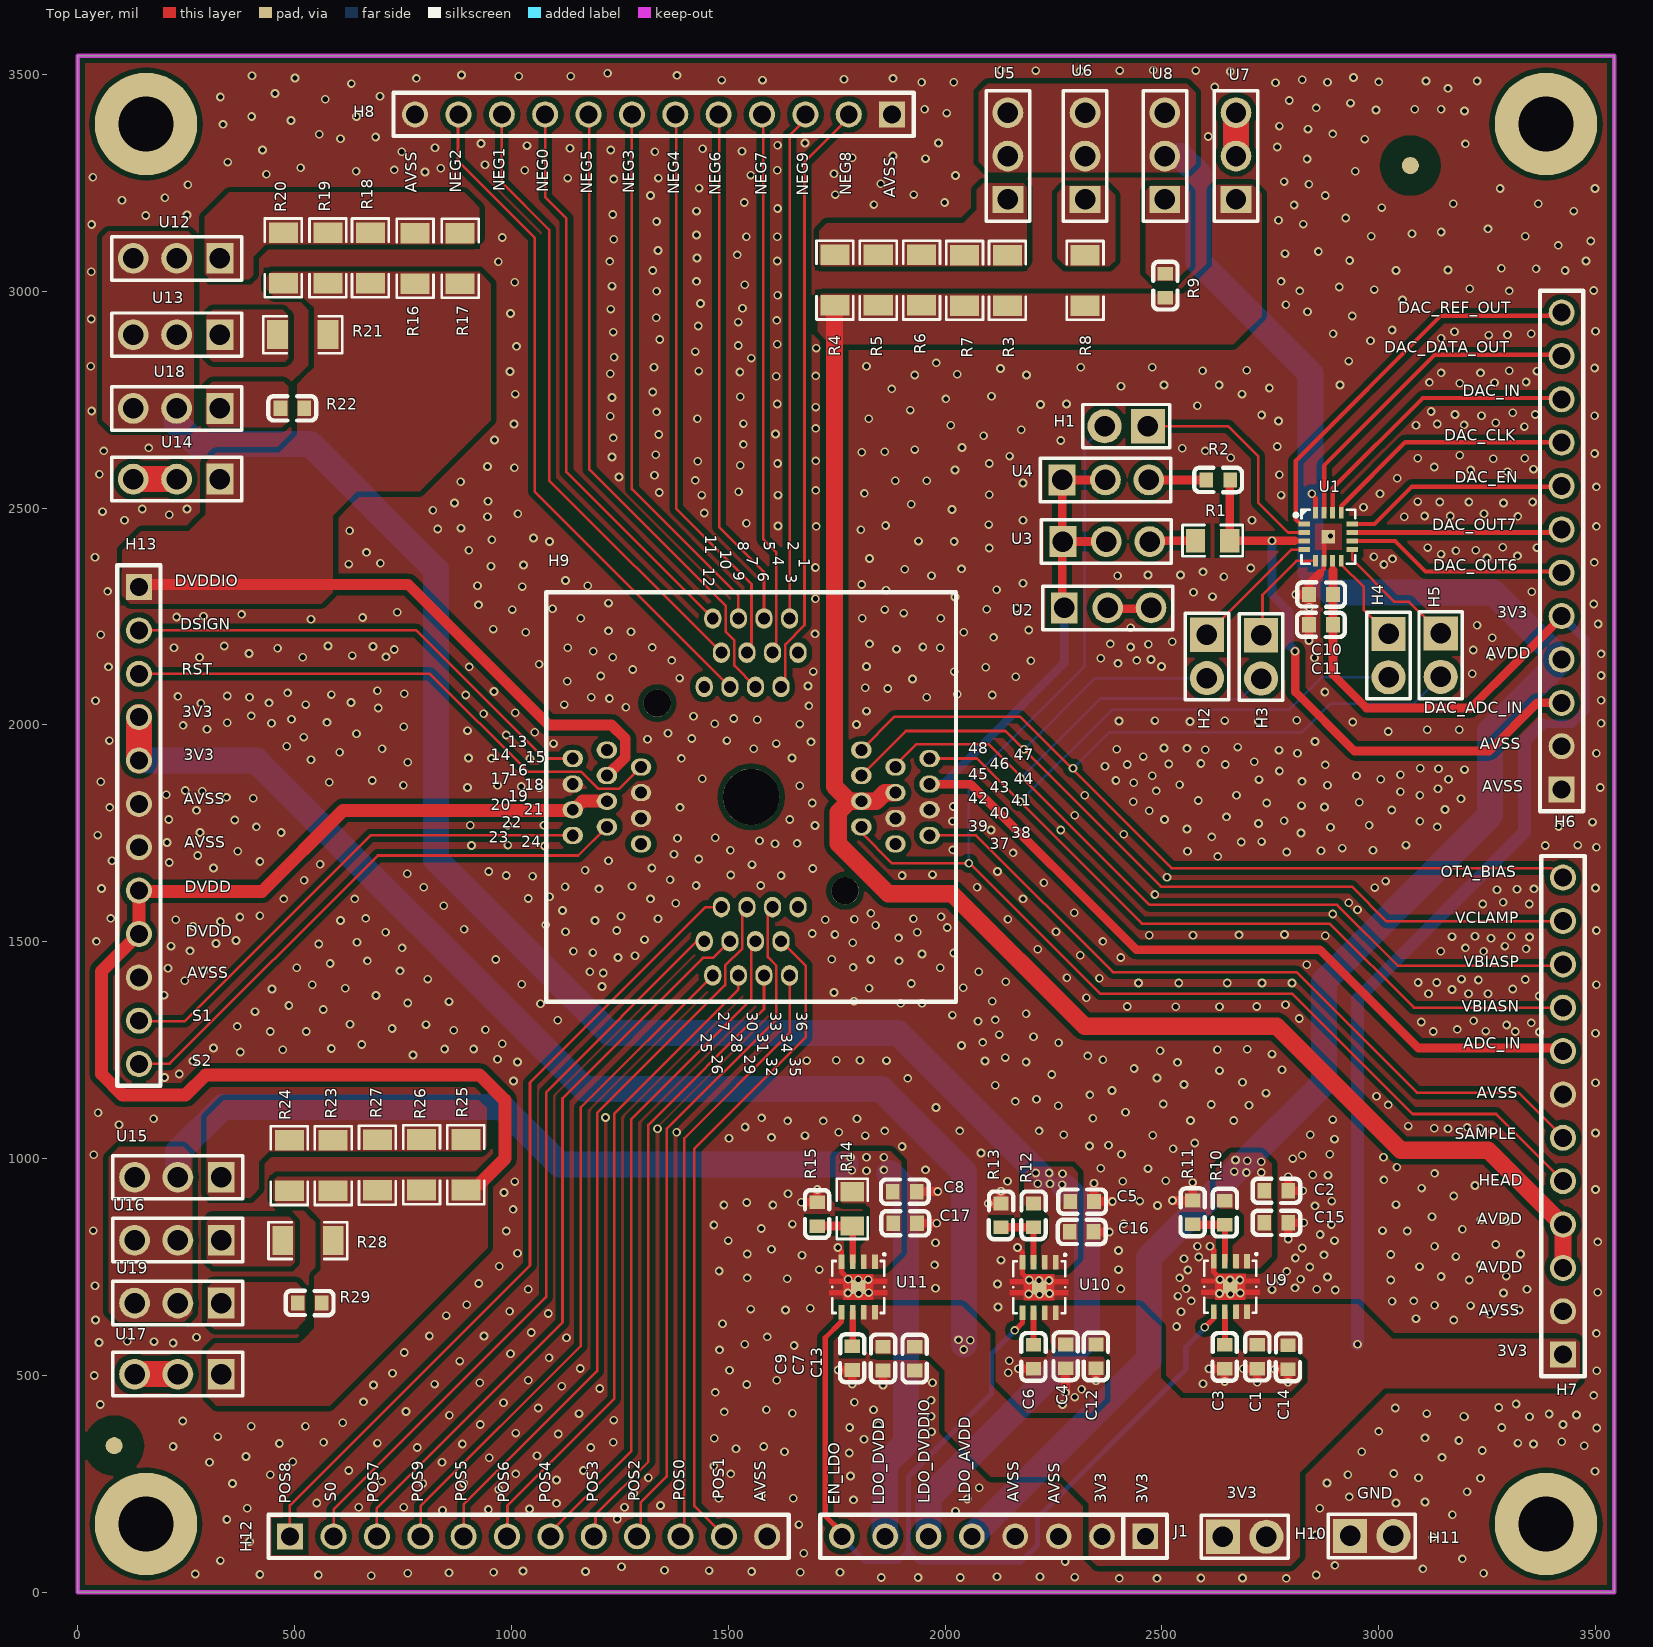
[diagram p0: Top Layer view]
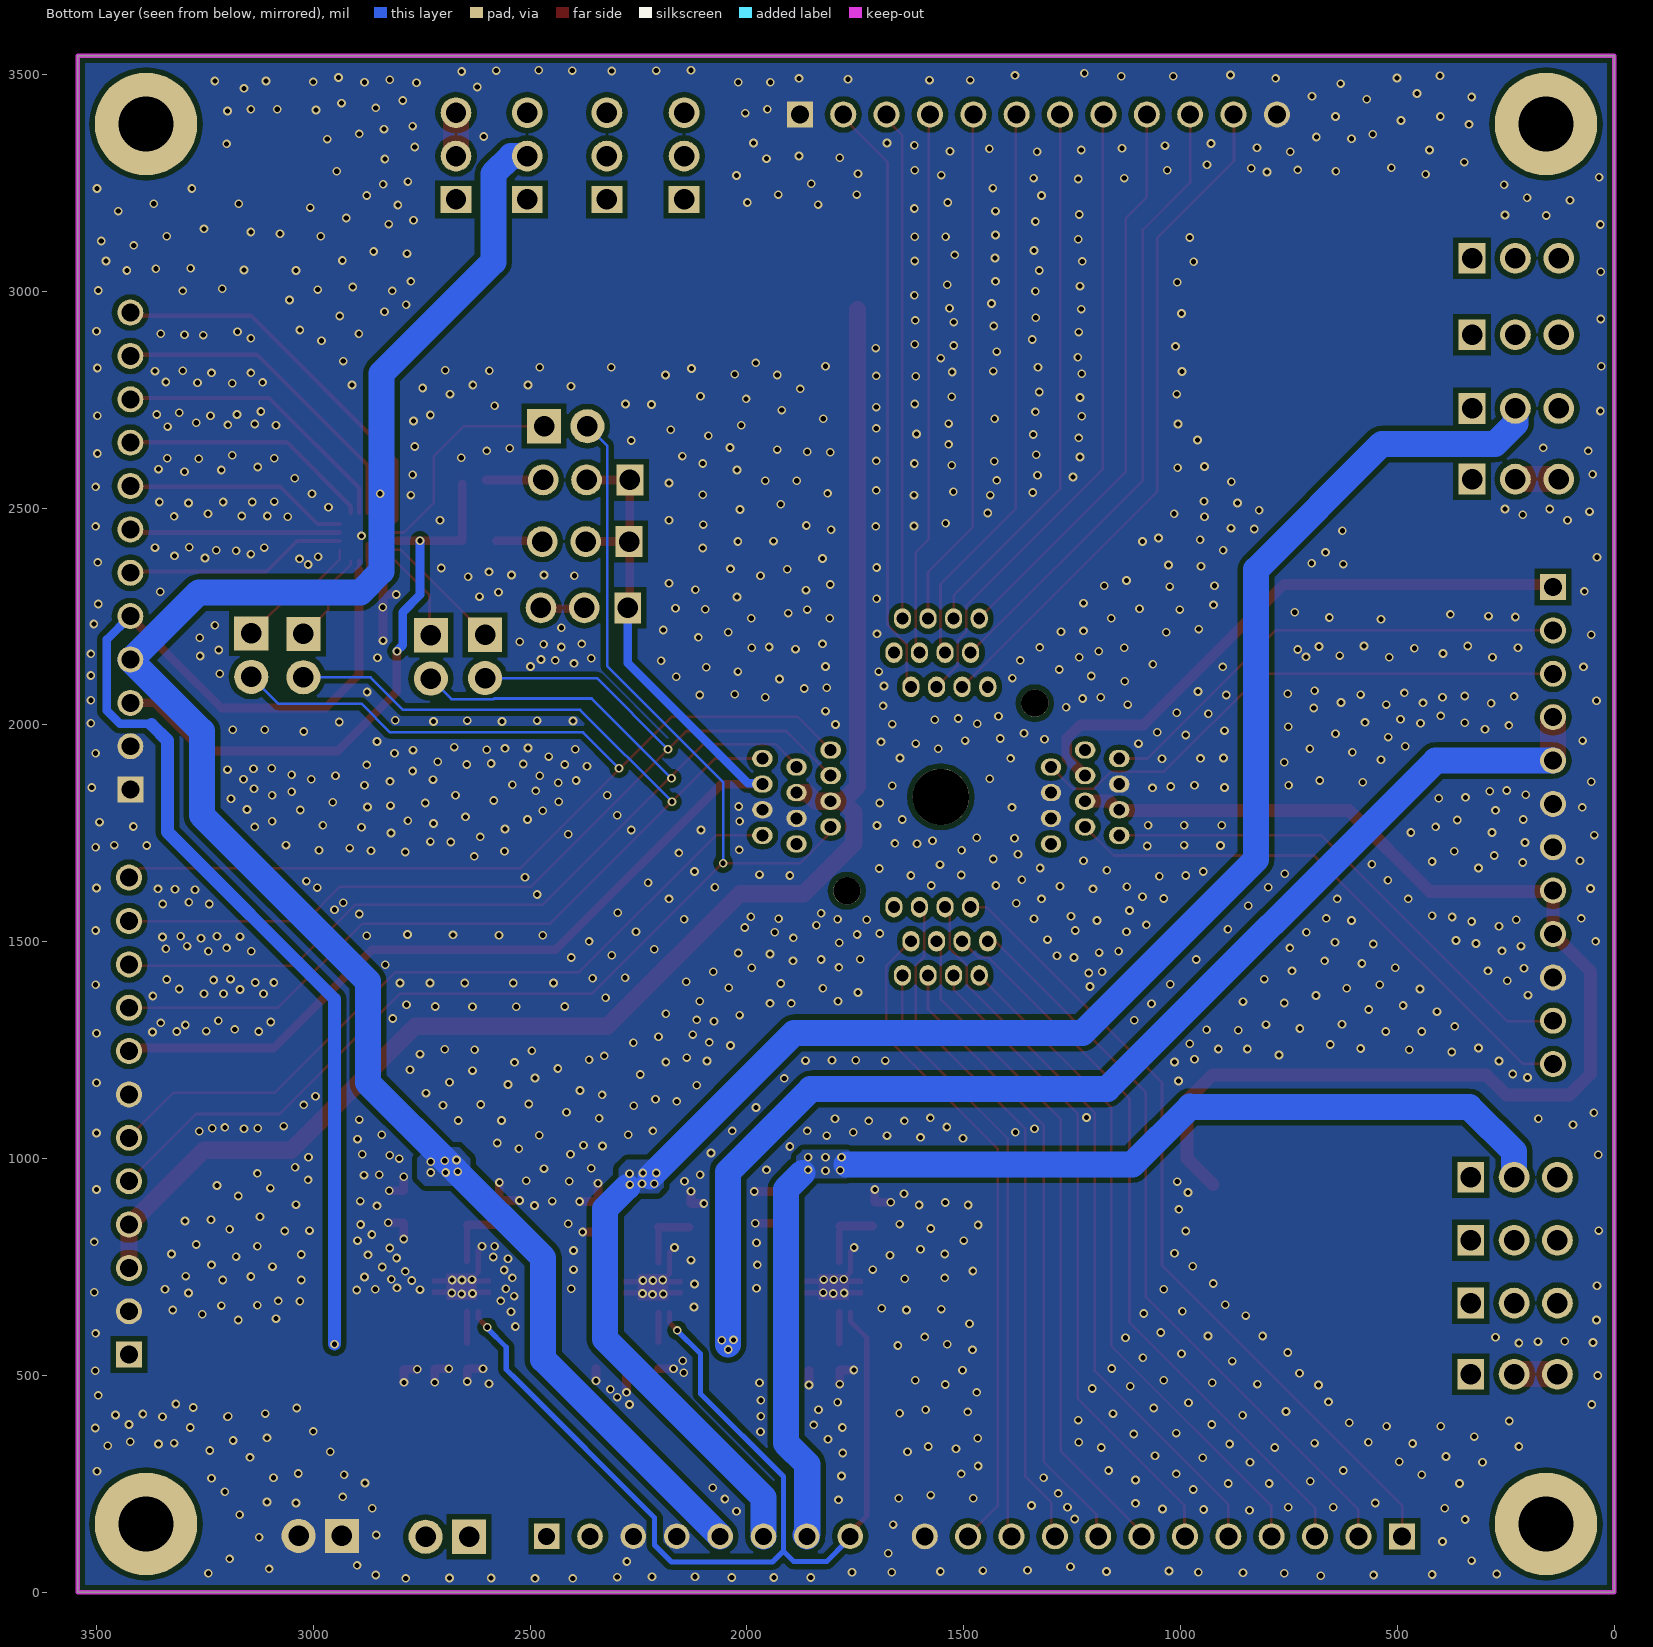
[diagram p1: Bottom Layer view, seen from below]
# Altium PCB MISC79022.pcbdoc (part 1 of 3)
Units mil, origin at the board's own origin, x right, y up, seen from the top; angles counter-clockwise.
Board outline 3543.31 x 3543.31 mil, 2 copper layers (Top Layer, Bottom Layer); 79 components, 75 nets, 320 pads, 1402 vias.

## Layer stack, top to bottom (the 12.6 mil dielectric is the usual default, probably not edited)
Top Layer: signal copper 1.4
Dielectric: dielectric 12.6, FR-4, Dk 4.8
Bottom Layer: signal copper 1.4

## Board outline
0,0 0,3543.31 3543.31,3543.31 3543.31,0

## Design rules (kind name [scope] priority, off if disabled: settings)
Clearance Clearance_2 [HASPAD('FREE-MARK')] p1: gap=50
Clearance Clearance_1 [INPOLYGON] p2: gap=6
Clearance [All] p3: gap=6
HoleSize [All] p1: absolutevalues=TRUE maxlimit=500 minlimit=1 maxpercent=80.000 minpercent=20.000
HoleToHoleClearance [All] p1: gap=0 allowstackedmicrovias=TRUE
MinimumSolderMaskSliver [All] p1: minsoldermaskwidth=0
PlaneConnect [All] p1: planeconnectstyle=Direct reliefexpansion=20 reliefentries=4 reliefconductorwidth=10 reliefairgap=10
PolygonConnect [All] p1: connectstyle=Direct reliefconductorwidth=10 reliefentries=4 polygonreliefangle="90 Angle"
RoutingVias [All] p1: holewidth=12 width=20 viastyle="Through Hole" minholewidth=12 minwidth=20 maxholewidth=12 maxwidth=20
SilkToSilkClearance [All] p1: silktosilkclearance=0
SilkscreenOverComponentPads [All] p1: minsilkscreentomaskgap=0
SolderMaskExpansion [All] p1: expansion=4
Width [All] p1: maxlimit=100 minlimit=6 preferedwidth=6 minimp=50.000000 maximp=50.000000 favimp=50.000000
22 further rules are at their usual default settings.

## Components (designator, comment, footprint, x,y, rotation, side; value= is the part's Value field where it differs from the comment)
C1 "1uF" C0603 2720,543 r270 top
C2 "4.7uF" C0603 2764,926 r180 top
C3 "10nF" C0603 2645,543 r90 top
C4 "1uF" C0603 2278,544 r270 top
C5 "4.7uF" C0603 2316,901 r180 top
C6 "10nF" C0603 2204,543 r90 top
C7 "1uF" C0603 1857,539 r270 top
C8 "4.7uF" C0603 1907,924 r180 top
C9 "10nF" C0603 1786,540 r90 top
C10 "1uF" C0603 2867.05,2301 r180 top
C11 "100nF" C0603 2867,2231 r0 top
C12 "4.7uF" C0603 2348,544 r90 top
C13 "4.7uF" C0603 1930,539 r90 top
C14 "4.7uF" C0603 2791,542 r90 top
C15 "4.7uF" C0603 2764,852 r180 top
C16 "4.7uF" C0603 2315,831 r180 top
C17 "4.7uF" C0603 1908,851 r180 top
H1 "PZ254V-11-02P" HDR-TH_2P-P2.54-V-M 2418,2689 r180 top
H2 "PZ254V-11-02P" HDR-TH_2P-P2.54-V-M 2604,2158 r270 top
H3 "PZ254V-11-02P" HDR-TH_2P-P2.54-V-M 2729,2157 r270 top
H4 "PZ254V-11-02P" HDR-TH_2P-P2.54-V-M 3023,2160 r270 top
H5 "PZ254V-11-02P" HDR-TH_2P-P2.54-V-M 3143,2161 r270 top
H6 "PZ254-1-12-Z-8.5" HDR-TH_12P-P2.54-V-M 3422,2401 r90 top
H7 "PZ254-1-12-Z-8.5" HDR-TH_12P-P2.54-V-M 3425,1098 r90 top
H8 "PZ254-1-12-Z-8.5" HDR-TH_12P-P2.54-V-M 1328,3408 r180 top
H9 "TQPF-48-Z" TQPF-48-Z 1553,1834 r270 top
H10 "PZ254V-11-02P" HDR-TH_2P-P2.54-V-M 2691,128 r0 top
H11 "PZ254V-11-02P" HDR-TH_2P-P2.54-V-M 2984,130 r0 top
H12 "PZ254-1-12-Z-8.5" HDR-TH_12P-P2.54-V-M 1040,129 r0 top
H13 "PZ254-1-12-Z-8.5" HDR-TH_12P-P2.54-V-M 141,1768 r270 top
J1 "Header2.54mm 1*8P" HDR-TH_8P-P2.54-V-M 2112,129 r180 top
R1 "100kΩ" R0805 2617,2425 r0 top
R2 "10.5kΩ" R0603 2630,2565 r0 top
R3 "10Ω" R1206 2144,3025 r270 top
R4 "10Ω" R1206 1746,3026 r270 top
R5 "10Ω" R1206 1846,3026 r270 top
R6 "10Ω" R1206 1946,3026 r270 top
R7 "10Ω" R1206 2045,3025 r270 top
R8 "10Ω" R1206 2323,3025 r270 top
R9 "118Ω" R0603 2508,3013 r270 top
R10 "12.6kΩ/1%" R0603 2645,875 r270 top
R11 "10kΩ/1%" R0603 2571,876 r270 top
R12 "12.6kΩ/1%" R0603 2204,869 r270 top
R13 "10kΩ/1%" R0603 2129,869 r270 top
R14 "1.25kΩ/1%" R0805 1786,884 r270 top
R15 "10kΩ/1%" R0603 1705,872 r270 top
R16 "10Ω" R1206 778,3076 r270 top
R17 "10Ω" R1206 882,3076 r270 top
R18 "10Ω" R1206 675,3077 r270 top
R19 "10Ω" R1206 577,3077 r270 top
R20 "10Ω" R1206 474,3077 r270 top
R21 "10Ω" R1206 519,2900 r0 top
R22 "118Ω" R0603 495,2730 r0 top
R23 "10Ω" R1206 589,984 r270 top
R24 "10Ω" R1206 488,984 r270 top
R25 "10Ω" R1206 895,986 r270 top
R26 "10Ω" R1206 793,986 r270 top
R27 "10Ω" R1206 691,985 r270 top
R28 "10Ω" R1206 531,811 r0 top
R29 "118Ω" R0603 535,667 r0 top
U1 "DAC60508ZRTER" WQFN-16_L3.0-W3.0-P0.50-BL-EP0.8 2884,2434 r270 top
U2 "2.54MM-1*3P 直针" HDR-TH_3P-P2.54-V-M-1 2375,2270 r0 top
U3 "2.54MM-1*3P 直针" HDR-TH_3P-P2.54-V-M-1 2372,2423 r0 top
U4 "2.54MM-1*3P 直针" HDR-TH_3P-P2.54-V-M-1 2370,2565 r0 top
U5 "2.54MM-1*3P 直针" HDR-TH_3P-P2.54-V-M-1 2145,3312 r90 top
U6 "2.54MM-1*3P 直针" HDR-TH_3P-P2.54-V-M-1 2323,3312 r90 top
U7 "2.54MM-1*3P 直针" HDR-TH_3P-P2.54-V-M-1 2671,3312 r90 top
U8 "2.54MM-1*3P 直针" HDR-TH_3P-P2.54-V-M-1 2507,3312 r90 top
U9 "TPS7A8001DRBR" VSON-8_L3.0-W3.0-P0.65-TL-EP 2657.95,705 r270 top
U10 "TPS7A8001DRBR" VSON-8_L3.0-W3.0-P0.65-TL-EP 2217,703 r270 top
U11 "TPS7A8001DRBR" VSON-8_L3.0-W3.0-P0.65-TL-EP 1800,704 r270 top
U12 "2.54MM-1*3P 直针" HDR-TH_3P-P2.54-V-M-1 228,3076 r180 top
U13 "2.54MM-1*3P 直针" HDR-TH_3P-P2.54-V-M-1 228,2900 r180 top
U14 "2.54MM-1*3P 直针" HDR-TH_3P-P2.54-V-M-1 228,2567 r180 top
U15 "2.54MM-1*3P 直针" HDR-TH_3P-P2.54-V-M-1 231,957 r180 top
U16 "2.54MM-1*3P 直针" HDR-TH_3P-P2.54-V-M-1 231,812 r180 top
U17 "2.54MM-1*3P 直针" HDR-TH_3P-P2.54-V-M-1 231,503 r180 top
U18 "2.54MM-1*3P 直针" HDR-TH_3P-P2.54-V-M-1 228,2730 r180 top
U19 "2.54MM-1*3P 直针" HDR-TH_3P-P2.54-V-M-1 231,667 r180 top

## Footprints (in the part's own frame and the unit in brackets; to place one, negate y for a bottom-side part, rotate by r counter-clockwise, add the part's x,y. Pads: shape width x height; smd on the part's side, far side on the other; paste and mask are expansions set on the pad)
C0603 [mm]
  rect 0.8x0.9 smd paste+0 mask+0.051: 1(-0.7,0) 2(0.7,0)
  silkscreen extent -1.41,-0.71 1.39,0.72
HDR-TH_2P-P2.54-V-M [mm]
  rect 2x2 hole 1.2 paste+0 mask+0.051: 1(-1.27,0)
  round 2 hole 1.2 paste+0 mask+0.051: 2(1.27,0)
  silkscreen extent -2.54,-1.27 2.54,1.27
HDR-TH_3P-P2.54-V-M-1 [mm]
  rect 1.575x1.8 hole 1.2 paste+0 mask+0.051: 1(-2.54,0)
  round 1.8 hole 1.2 paste+0 mask+0.051: 2(0,0) 3(2.54,0)
  silkscreen extent -3.81,-1.27 3.81,1.27
HDR-TH_8P-P2.54-V-M [mm]
  rect 1.5x1.5 hole 1 paste+0 mask+0.051: 1(-8.89,0)
  round 1.5 hole 1 paste+0 mask+0.051: 2(-6.35,0) 3(-3.81,0) 4(-1.27,0) 5(1.27,0) 6(3.81,0) 7(6.35,0) 8(8.89,0)
  silkscreen extent -10.16,-1.27 10.16,1.27
HDR-TH_12P-P2.54-V-M [mil]
  rect 60x60 hole 41.34 paste+0 mask+2: 1(-550,0)
  round 60 hole 41.34 paste+0 mask+2: 2(-450,0) 3(-350,0) 4(-250,0) 5(-150,0) 6(-50,0) 7(50,0) 8(150,0) 9(250,0) 10(350,0) 11(450,0) 12(550,0)
  silkscreen extent -600,-50 600,50
R0603 [mm]
  rect 0.8x0.9 smd paste+0 mask+0.051: 1(-0.7,0) 2(0.7,0)
  silkscreen extent -1.41,-0.71 1.39,0.72
R0805 [mil]
  rect 44.59x54.21 smd paste-3937.01 mask+2: 1(-39.37,0) 2(39.37,0)
  silkscreen extent -69,-36 69,36
R1206 [mil]
  rect 47.54x66.97 smd paste-3937.01 mask+2: 1(-58.22,0) 2(58.22,0)
  silkscreen extent -91,-42 91,42
TQPF-48-Z [mm]
  round 1.6 hole 1.6 unplated: 0(-5.5,-5.5) 0(5.5,5.5)
  round 3.3 hole 3.3 unplated: 0(0,0)
  oval 1.2x1 hole 0.7: 1(-8.45,2.75) 2(-10.45,2.25) 3(-6.45,1.75) 4(-8.45,1.25) 5(-10.45,0.75) 6(-6.45,0.25) 7(-8.45,-0.25) 8(-10.45,-0.75) 9(-6.45,-1.25) 10(-8.45,-1.75) 11(-10.45,-2.25) 12(-6.45,-2.75) 25(8.45,-2.75) 26(10.45,-2.25) 27(6.45,-1.75) 28(8.45,-1.25) 29(10.45,-0.75) 30(6.45,-0.25) 31(8.45,0.25) 32(10.45,0.75) 33(6.45,1.25) 34(8.45,1.75) 35(10.45,2.25) 36(6.45,2.75)
  oval 1x1.2 hole 0.7: 13(-2.75,-8.45) 14(-2.25,-10.45) 15(-1.75,-6.45) 16(-1.25,-8.45) 17(-0.75,-10.45) 18(-0.25,-6.45) 19(0.25,-8.45) 20(0.75,-10.45) 21(1.25,-6.45) 22(1.75,-8.45) 23(2.25,-10.45) 24(2.75,-6.45) 37(2.75,8.45) 38(2.25,10.45) 39(1.75,6.45) 40(1.25,8.45) 41(0.75,10.45) 42(0.25,6.45) 43(-0.25,8.45) 44(-0.75,10.45) 45(-1.25,6.45) 46(-1.75,8.45) 47(-2.25,10.45) 48(-2.75,6.45)
  silkscreen extent -12,-12 12,12
VSON-8_L3.0-W3.0-P0.65-TL-EP [mm]
  rect 0.85x0.34 smd paste+0 mask+0.051: 1(-1.476,0.975) 2(-1.476,0.325) 3(-1.476,-0.325) 4(-1.476,-0.975) 5(1.476,-0.975) 6(1.476,-0.325) 7(1.476,0.325) 8(1.476,0.975)
  rect 0.838x0.838 smd paste+0 mask+0.051: 9(0,0)
  Top Layer region: -0.76,0.89 -0.47,0.89 -0.47,1.71 -0.18,1.71 -0.18,0.88 0.18,0.88 0.18,1.71 0.47,1.71 0.47,0.88 0.76,0.88 0.76,-0.89 0.47,-0.89 0.47,-1.71 0.18,-1.71 0.18,-0.89 -0.18,-0.89 -0.18,-1.71 -0.47,-1.71 -0.47,-0.89 -0.76,-0.89 -0.76,0.89
  silkscreen extent -1.96,-1.52 1.52,1.58
WQFN-16_L3.0-W3.0-P0.50-BL-EP0.8 [mm]
  rect 0.28x0.665 smd paste+0 mask+0.051: 1(-0.75,-1.407) 2(-0.25,-1.407) 3(0.25,-1.407) 4(0.75,-1.407) 9(0.75,1.407) 10(0.25,1.407) 11(-0.25,1.407) 12(-0.75,1.407)
  rect 0.665x0.28 smd paste+0 mask+0.051: 5(1.407,-0.75) 6(1.407,-0.25) 7(1.407,0.25) 8(1.407,0.75) 13(-1.407,0.75) 14(-1.407,0.25) 15(-1.407,-0.25) 16(-1.407,-0.75)
  rect 0.8x0.8 smd paste+0 mask+0.051: 17(0,0)
  silkscreen extent -1.58,-2 1.58,1.58

## Part data
C11: library part 10nF
H9: library part PZ254-1-12-Z-8.5

## Free pads (board coordinates)
  round 236.22 hole 125.98: 0(157.48,157.48) 0(157.48,3385.83) 0(3385.83,157.48) 0(3385.83,3385.83)
  round 39.37 smd mask+39.37: MARK(84,338) MARK(3073,3290)

## Via types
v1: diameter 20, hole 12, Top Layer to Bottom Layer, 1402 vias

## Nets (pads, with @x,y where several pads share a name; then routed paths per layer and width w, separated by ;. In a path a pad name is that pad's centre, name@x,y a point inside that pad or via, vN(x,y) a via of type N, cw(c..) or ccw(c..) an arc to the next point about the centre after c; other vN are vias at no path point)
3.3V: C1.1 C4.1 C7.1 C10.1 C11.2 C12.2 C13.2 C14.2 H6.5 H7.1 H10.1 H10.2 H13.4 H13.5 J1.1 J1.2 U1.7 U9.7 U9.8 U10.7 U10.8 U11.7 U11.8 | length 5668.5
  Top Layer w11: 2893.84,2356.33 U1.7@2893.84,2378.59
  Top Layer w20: 2894.56,2356.33 C11.2@2894.56,2231 2894.56,2116.44 2972,2039 3212,2039 3316,2143 ; 3325,2152 3316,2143 ; H6.5@3417,2244 3316,2143
  Top Layer w60: H13.5@141,1918 H13.4@141,2018
  Bottom Layer w20: 3372.5,2001.5 3374,2003 3446,2003 3476,2033 3476,2197 H6.5@3422,2251
  Bottom Layer w30: v1(2951,572) 2951,1368 3336,1753 3336,1964 3373,2001
  Bottom Layer w60: H13.5@141,1918 412,1918 1169,1161 1850,1161 1852,1159 ; 1853,1160 2044,969 2044,571
  other v1: 2043,560 2058,581 2031,582
ADC_IN: H7.8 H9.44 U2.1 U3.1 U3.2 U4.1 U4.2 | length 2764.4
  Top Layer w20: H9.44@1964.42,1863.53 2059.47,1863.53 2441,1482 2864,1482 3091,1255 H7.8@3428,1255 ; U3.1@2261,2423 U3.1@2272,2423 U3.2@2372,2423 ; U4.1@2268,2565 U4.1@2270,2565 ; U2.1@2270,2283 2270,2335 U4.1@2270,2565 ; U4.2@2370,2565 U4.1@2270,2565
  Bottom Layer w20: H9.44@1963,1866 1998,1866 2275,2143 U2.1@2275,2270
AVDD: H7.3 H7.4 H9.42 H9.43 R3.2 R4.2 R5.2 R6.2 R7.2 R8.2 R9.2 U7.1 | length 3496.4
  Top Layer w40: R4.2@1745,2958 1745,1858.31 1779.16,1824.16 ; H9.42@1804,1824 1841,1824 1860.84,1843.84 H9.43@1885.68,1843.84 ; H9.42@1806.94,1824.16 1779.16,1824.16 ; H7.4@3418,848 H7.4@3423,848 ; H7.4@3418,854 3253,1019 3051,1019 2765,1305 2322,1305 2016,1611 1869,1611 1754,1726 1754,1799 1779.16,1824.16 ; H7.3@3425,756 H7.4@3425,848
AVDD_CUR_IN: U7.2 U7.3 | length 85
  Top Layer w60: U7.2@2671,3312 U7.3@2671,3397